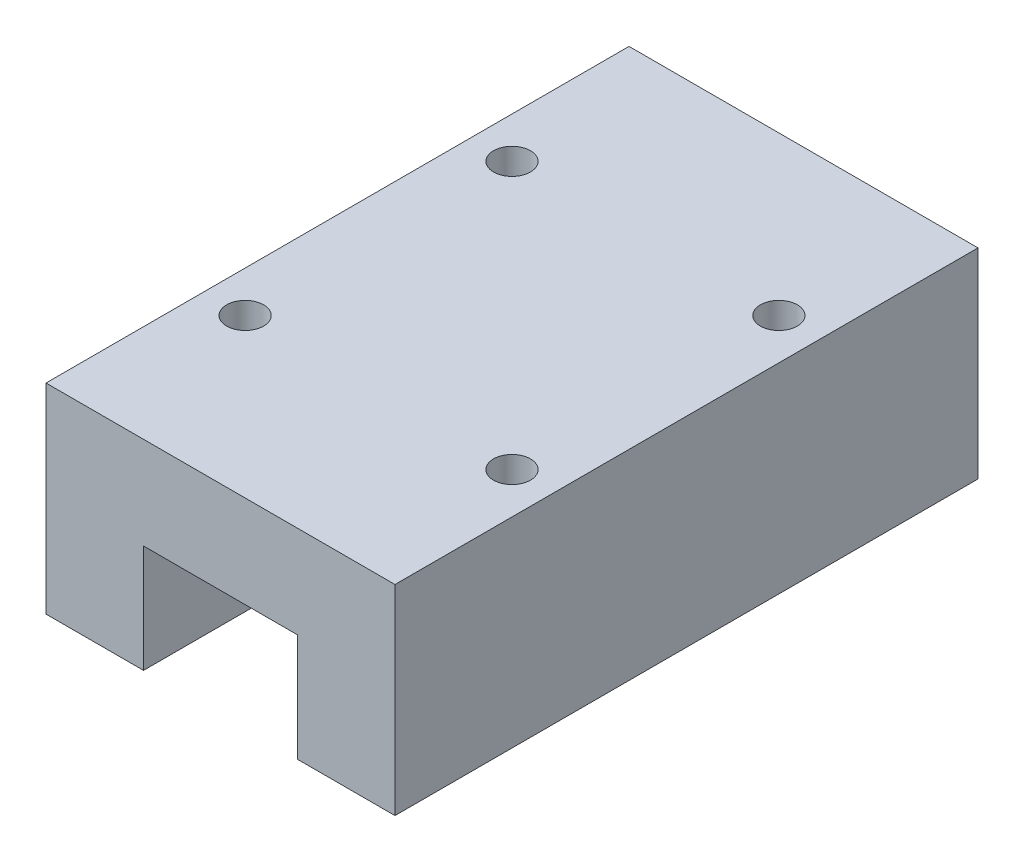
SolidWorks part; units mm, degrees
material "普通碳钢"
ref_plane "前视基准面" through (0, 0, 0) normal (0, 0, 1) x (1, 0, 0)
ref_plane "上视基准面" through (0, 0, 0) normal (0, 1, 0) x (1, 0, 0)
ref_plane "右视基准面" through (0, 0, 0) normal (1, 0, 0) x (0, 0, -1)
sketch "草图1" plane through (0, 0, 0) normal (0, 0, 1) x (1, 0, 0)
  line L1 (-17, 9.75) -> (17, 9.75)
  line L2 (-17, 9.75) -> (-17, -9.75)
  line L3 (-17, -9.75) -> (17, -9.75)
  line L4 (17, 9.75) -> (17, -9.75)
  line L5 (-17, 9.75) -> (17, -9.75) construction
  line L6 (-17, -9.75) -> (17, 9.75) construction
  point P0 (0, 0)
  dimension "D1" = 19.5
  dimension "D2" = 34
extrude "凸台-拉伸1" add sketch "草图1" along normal mid plane 56.8
sketch "草图2" plane through (0, 0, 0) normal (0, 0, 1) x (1, 0, 0)
  line L0 (0, 0) -> (0, -9.75) construction
  line L1 (-17, -9.75) -> (17, -9.75) construction
  line L3 (-7.5, 0.75) -> (7.5, 0.75)
  line L4 (-7.5, 0.75) -> (-7.5, -9.75)
  line L5 (-7.5, -9.75) -> (7.5, -9.75)
  line L6 (7.5, 0.75) -> (7.5, -9.75)
  line L7 (-7.5, 0.75) -> (7.5, -9.75) construction
  line L8 (-7.5, -9.75) -> (7.5, 0.75) construction
  point P5 (0, -4.5)
  dimension "D1" = 15
  dimension "D2" = 10.5
extrude "切除-拉伸1" cut sketch "草图2" against normal through all both and the other way through all
sketch "草图4" plane through (0, 9.75, 0) normal (0, 1, 0) x (1, 0, 0)
  line L0 (0, 28.4) -> (0, -28.4) construction
  line L1 (17, 28.4) -> (-17, 28.4) construction
  line L2 (17, -28.4) -> (-17, -28.4) construction
  line L3 (-17, 0) -> (17, 0) construction
  line L4 (-17, -28.4) -> (-17, 28.4) construction
  line L5 (17, -28.4) -> (17, 28.4) construction
  circle A0 centre (-13, 13) radius 1.8
  circle A1 centre (13, 13) radius 1.8
  circle A2 centre (13, -13) radius 1.8
  circle A3 centre (-13, -13) radius 1.8
  dimension "D2" = 3.6
  dimension "D1" = 26
  dimension "D3" = 26
extrude "切除-拉伸2" cut sketch "草图4" against normal blind 6
